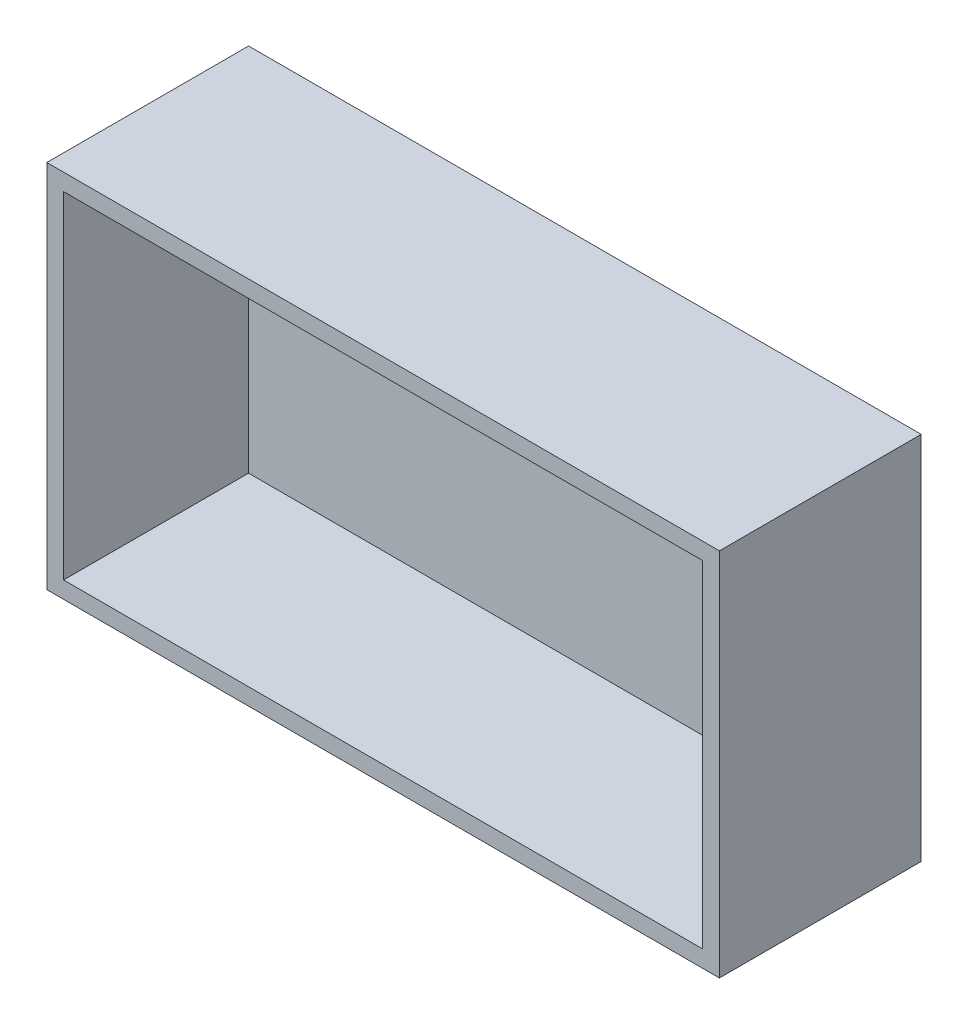
from build123d import *

# Parameters (mm, degrees)
SKETCH_1_W      = 400
SKETCH_1_H      = 220
SKETCH_1_W_2    = 380
SKETCH_1_H_2    = 200
EXTRUDE_1_DEPTH = 120
SKETCH_2_W      = 400
SKETCH_2_H      = 10
EXTRUDE_2_DEPTH = 210


with BuildPart() as part:
    # 草图1 → 拉伸-薄壁1 (new body)
    with BuildSketch(Plane.XY):
        Rectangle(SKETCH_1_W, SKETCH_1_H)
        Rectangle(SKETCH_1_W_2, SKETCH_1_H_2, mode=Mode.SUBTRACT)
    extrude(amount=EXTRUDE_1_DEPTH)

    # 草图2 → 凸台-拉伸2 (add)
    with BuildSketch(Plane(origin=(0, 100, 0), x_dir=(-1, 0, 0), z_dir=(0, -1, 0))):
        with Locations((0, -5)):
            Rectangle(SKETCH_2_W, SKETCH_2_H)
    extrude(amount=EXTRUDE_2_DEPTH)


solid = part.part
